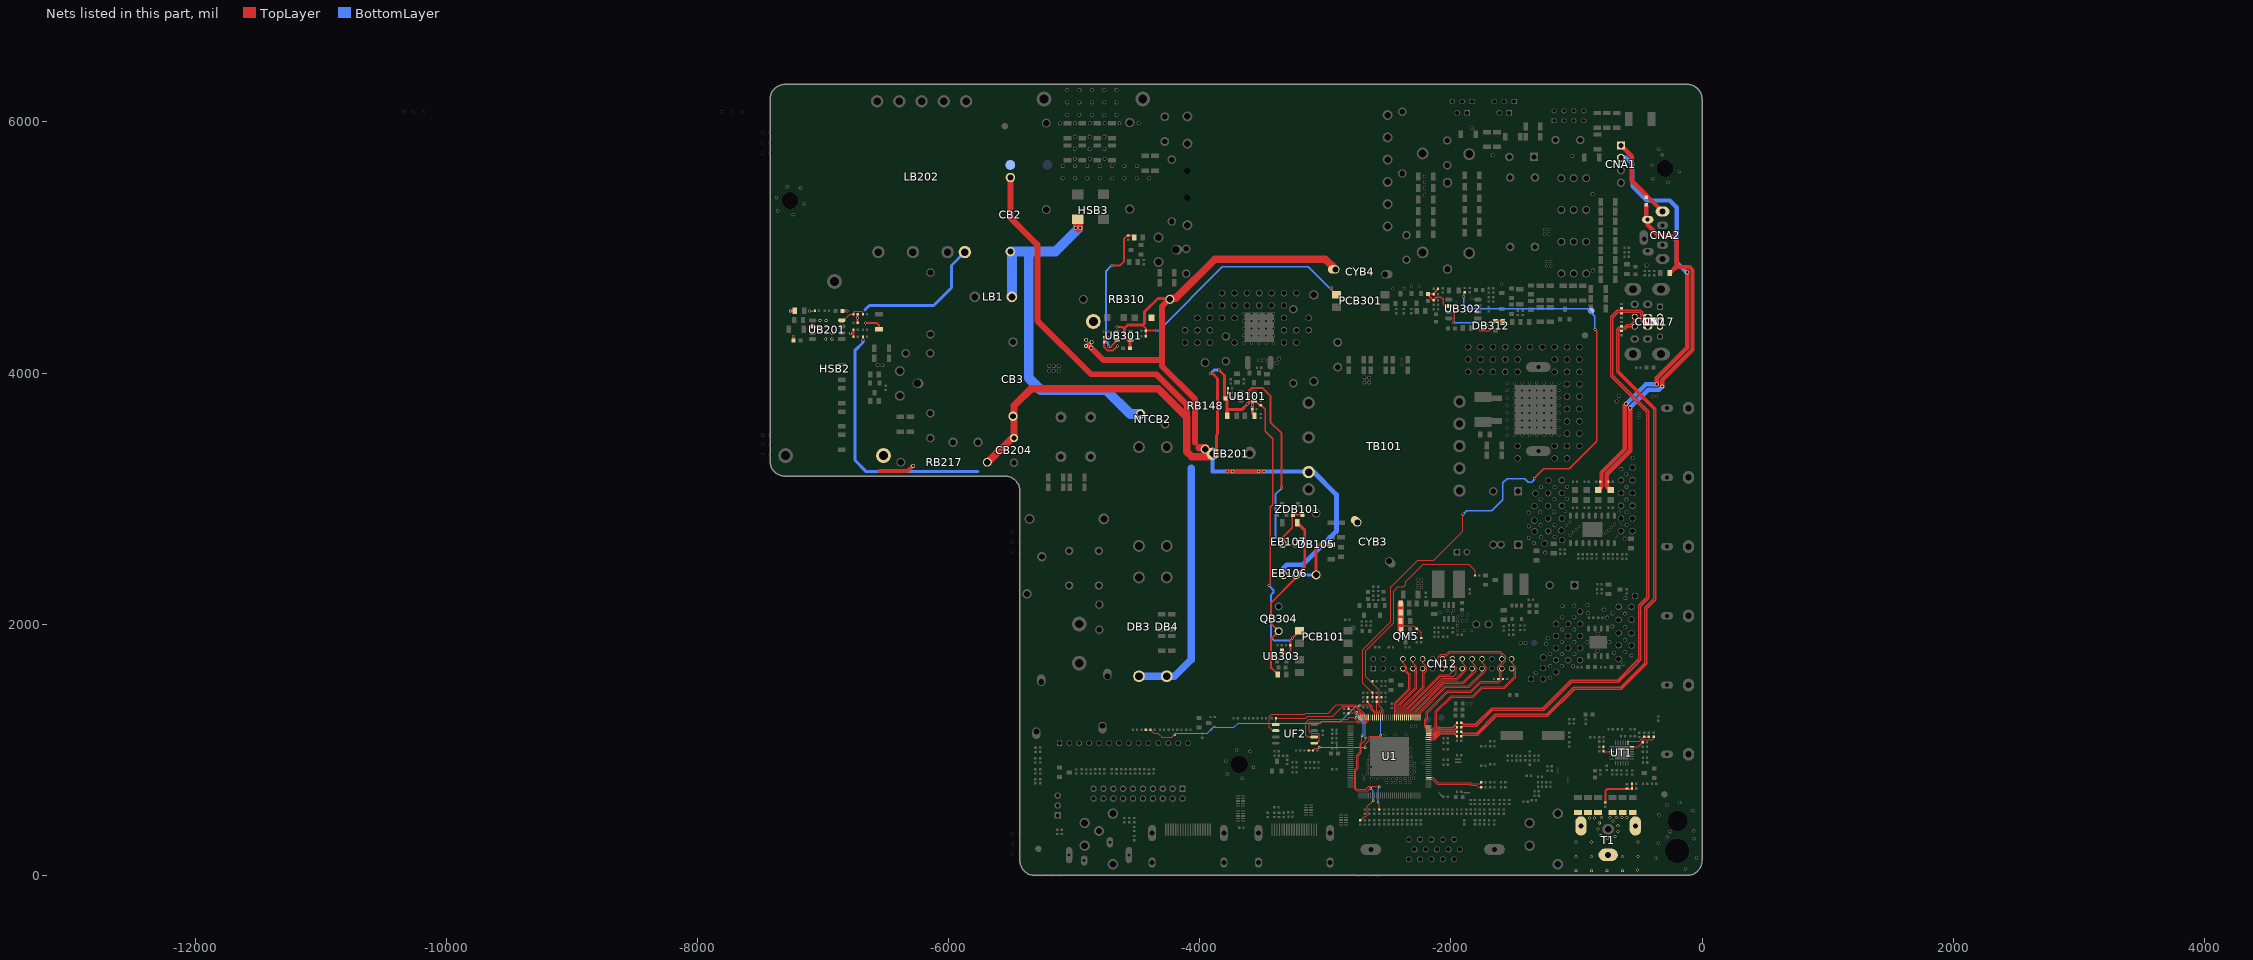
[diagram p0: the nets of this part, all layers, seen from the top]
# Altium PCB MISC84277.PcbDoc (part 13 of 15)
Units mil, origin at the board's own origin, x right, y up, seen from the top; angles counter-clockwise.
Board outline 7422.08 x 6299.21 mil, 2 copper layers (TopLayer, BottomLayer), stack 61.855 mil thick; 709 components, 395 nets, 2812 pads, 811 vias.

## Via types
v1: diameter 23.62, hole 15.75, TopLayer to BottomLayer, tented both sides, 437 vias
v2: diameter 19.68, hole 11.81, TopLayer to BottomLayer, tented both sides, 353 vias
v3: diameter 31.5, hole 23.62, TopLayer to BottomLayer, tented both sides, 16 vias
v4: diameter 31.5, hole 19.68, TopLayer to BottomLayer, tented both sides, 4 vias
v5: diameter 17.72, hole 9.84, TopLayer to BottomLayer, tented both sides, 1 vias

## Nets (pads, with @x,y where several pads share a name; then routed paths per layer and width w, separated by ;. In a path a pad name is that pad's centre, name@x,y a point inside that pad or via, vN(x,y) a via of type N, cw(c..) or ccw(c..) an arc to the next point about the centre after c; other vN are vias at no path point) (continued)
OUT: RB306.1 RB307.1 UB301.6 | length 1145.5
  TopLayer w15.75: v1(-4726.37,4210.62) -4724.41,4208.66 -4709.38,4208.66 UB301.6@-4658.19,4259.84 ; v1(-4700.79,4858.27) -4633.86,4858.27 -4602.36,4889.76 -4602.36,5071.02 RB307.1@-4577.15,5096.23 ; RB307.1@-4569.47,5096.23 -4540.8,5096.23 RB306.1@-4524.06,5079.5
  BottomLayer w15.75: v1(-4726.37,4210.62) -4726.37,4224.4 -4746.06,4244.09 -4746.06,4812.99 v1(-4700.79,4858.27)
OVP: CB322.2 CB323.2 CB324.2 CB328.1 DB312.2 RB351.2 UB302.6 | length 999.2
  TopLayer w11.81: CB322.2@-2177.81,4630.31 CB322.2@-2184,4630.31 ; CB323.2@-2137.23,4629.5 CB323.2@-2137.23,4632.9 ; CB323.2@-2136.73,4632.9 CB323.2@-2137.23,4632.9 ; RB351.2@-2103.84,4668.53 -2137.23,4635.13 CB323.2@-2137.23,4632.9 ; UB302.6@-2046.5,4536 -2062.84,4552.34 -2062.84,4587.34 -2080.25,4604.75 -2117.39,4604.75 -2136.23,4585.9 CB324.2@-2136.23,4581 -2139.15,4581 -2184,4625.85 CB322.2@-2184,4630.31 ; UB302.6@-2017.56,4536 -1991.5,4536 -1974.13,4518.63 -1974.13,4407.87 v1(-1980,4402) ; v1(-1780,4401.5) -1780,4350.5 -1768,4338.5 -1695.5,4338.5 -1680,4354 -1680,4380 DB312.2@-1645.5,4414.5 -1643,4417 -1596.03,4417 CB328.1@-1586.53,4407.5 ; CB322.2@-2184,4630.31 -2181.41,4632.9 CB323.2@-2137.23,4632.9
  BottomLayer w11.81: v1@-1979.66,4402.34 v1@-1780.84,4402.34
PC_LIN: CV6.2 U1.38 | length 444.7
  TopLayer w7: U1.38@-2178.42,781.32 -2145.35,781.32 -2100.56,736.53 -1839.56,736.53 -1833.53,730.5 -1768.23,730.5 CV6.2@-1758.73,739.99
PC_RIN: CV5.2 U1.37 | length 451.4
  TopLayer w7: U1.37@-2178.42,765.57 -2148.57,765.57 -2107.53,724.53 -1844.53,724.53 -1838.5,718.5 -1797.28,718.5 -1779.78,701 CV5.2@-1758.73,701 ; CV5.2@-1761,701 CV5.2@-1758.73,701 ; CV5.2@-1758.73,703.73 CV5.2@-1758.73,701
PFC_CS: CB205.2 RB215.1 UB201.4 | length 225.8
  TopLayer w7.87: UB201.4@-6851.71,4420.37 -6834.63,4420.37 -6786.21,4468.79 CB205.2@-6757.93,4468.79 -6757.93,4482.57 -6747.5,4493 -6692,4493 -6683.12,4484.12 RB215.1@-6683.12,4468.8
PVCC: CM3.2 CM5.2 QM5.S R5V.2 R12V.2 RM5.2 | length 440
  TopLayer w6: -2397.94,1988.24 -2297.24,1988.24 -2272.73,1963.73 -2267.73,1963.73 -2235,1931 RM5.2@-2235,1890.73
  TopLayer w50: R12V.2@-2399.61,2165.35 QM5.S@-2399.4,1952.24
PWM0: RF13.1 RG2.1 U1.86 | length 165.6
  TopLayer w6: RG2.1@-2591.27,1417 -2591.27,1307.54 -2576.05,1292.32 U1.86@-2576.05,1257.7
PWM1: RF18.1 RG1.2 U1.87 | length 191
  TopLayer w6: RG1.2@-2665.27,1417 -2665.27,1384.27 -2627,1346 -2627,1325.56 -2591.8,1290.36 U1.87@-2591.8,1257.7 U1.87@-2590.89,1258.61
PWM_REF: CG2.1 PWM_REF.1 RB366.2 RG2.2 | length 5499.1
  TopLayer w6: RG2.2@-2624.73,1417 CG2.1@-2624.73,1454 -2627,1454 -2701.27,1528.27 -2701.27,1798.4 -2479,2020.67 -2479,2295.92 -2264.92,2510 -2137.83,2510 -1905.51,2742.32 v1(-1905.51,2875.98)
  TopLayer w11.81: v1(-1898.5,4610) -1898.5,4634.27 RB366.2@-1889,4643.77 ; v1(-1336.61,3161.41) -1259.83,3238.19 -1058.78,3238.19 -838.59,3458.39 -838.59,4332.68 v1(-854.33,4348.43)
  BottomLayer w11.81: v1(-1905.51,2875.98) -1875.9,2905.6 -1674.2,2905.6 -1588.1,2991.7 -1588.1,3125.8 -1553.6,3160.3 -1412.8,3160.3 -1382.8,3130.3 -1356.3,3130.3 -1336.61,3149.99 v1(-1336.61,3161.41) ; v1(-1898.5,4610) -1898.5,4547.11 -1864.21,4512.82 -914.39,4512.82 -854.33,4452.76 v1(-854.33,4348.43)
PWR_ON/OFF: RM3.2 RM4.2 RM8.1 U1.84 | length 1985.9
  TopLayer w6: -2572,1417 RM3.2@-2553.73,1417 ; U1.84@-2544.56,1257.7 -2544.56,1287.26 -2540.27,1291.54 -2540.27,1316.27 -2573,1349 -2573,1476 -2679.27,1582.27 -2679.27,1789.29 -2457,2011.56 -2457,2263.47 -2423.32,2297.15 -2376.08,2297.15 -2360.24,2312.99 -2360.24,2336.42 -2219.66,2477 -1859,2477 -1807.73,2425.73 RM4.2@-1807.73,2388
REMOTE: CK6.2 RK16.1 U1.88 | length 2045.2
  TopLayer w6: RK16.1@-4431.56,1160.01 CK6.2@-4393.63,1160.01 -4366.72,1133.1 -4336.05,1133.1 -4301.05,1098.1 -4222.7,1098.1 v2(-4201.3,1119.5) ; v2(-2729,1351) -2721,1359 -2655.56,1359 -2638,1341.44 -2638,1321 -2607.55,1290.55 U1.88@-2607.55,1257.7 U1.88@-2608.3,1258.45
  BottomLayer w6: v2(-4201.3,1119.5) -4189.13,1131.67 -4034.1,1131.67 ; -4047.3,1131.67 -4034.1,1131.67 ; v2(-2729,1351) -2756,1351 -2879,1228 -3027.36,1228 -3042.36,1213 -3695.6,1213 -3730.24,1178.36 -3893.19,1178.36 -3939.87,1131.67 -4034.1,1131.67
RESET-H: U1.89 | length 0.9
  TopLayer w6: U1.89@-2623.3,1257.7 U1.89@-2622.66,1258.34
RF_INPUT: CT13.1 CT40.2 LT3.1 LT11.1 | length 350.1
  TopLayer w15.8: CT40.2@-770.21,579.99 -770.21,662.29 cw(c-741.83,662.29) -761.9,682.36 cw(c-744.86,665.32) -744.86,689.41 -560.31,689.41 LT3.1@-557.46,692.26 CT13.1@-557.46,730.28
RFGND: CT41.2 CT42.2 CT43.2 CT44.2 CT45.2 CT46.2 T1.2 T1.3 T1.4
  other v1: -1006,36.65 -881.75,36.65 -757.5,36.65 -633.25,36.65 -515,41 -1006,152 -881.75,152 -633.25,152 -509,152 -1006,267.35 -881.75,267.35 -509,267.35 -753,295 -695,310 -807,316 -669,348 -830,369 -670,395 -815,418 -708,434 -898,457 -857,458 -801,459 -682,460 -639,460 -598,460 -734,461
ROUT+: CA10.1 CA40.2 CNA2.4 LBA4.2 pad.VIA5@-317.13,3893.19 pad.VIA5@-572.38,3725.25 RA17.1 | length 2944.6
  TopLayer w35: -759,3134.02 -759,3099 LBA4.2@-728,3068 ; -759,3137 -759,3194 -571.5,3381.5 pad.VIA5@-571.5,3723.5 ; CNA2.4@-444.88,5226.4 RA17.1@-444.88,5333.9 ; CNA2.4@-433.07,5222.44 -433.07,5180.2 -348.87,5096 -244.09,5096 -200.89,5052.79 -200.89,4851.88 CA40.2@-256.26,4796.5 ; pad.VIA5@-317.13,3893.19 -317.13,3944.09 -76,4185.22 -76,4821.5 -99.5,4845 -200.89,4845
  BottomLayer w35: pad.VIA5@-572.38,3725.25 -429.63,3868 -342.31,3868 pad.VIA5@-317.13,3893.19
ROUT+': CNA1.1 CNA2.6 RA17.2 | length 678.2
  TopLayer w35: CNA1.1@-646.5,5799.2 CNA1.1@-646.5,5813.67 -560,5727.17 -560,5652.29 -559.5,5651.79 -559.5,5531.5 CNA2.6@-319.34,5291.34
  TopLayer w40: CNA2.6@-319.34,5291.34 CNA2.6@-314.96,5291.34
  BottomLayer w40: CNA2.6@-314.96,5291.49 CNA2.6@-314.96,5293
ROUT-: CA17.1 CNA1.2 LBA3.2 pad.VIA5@-119,4802 pad.VIA5@-360.13,3911 pad.VIA5@-602.2,3756.25 | length 3413.4
  TopLayer w35: LBA3.2@-827,3068 -801,3094 -801,3208.57 -614.5,3395.07 -614.5,3743.94 pad.VIA5@-602.26,3756.19 ; pad.VIA5@-360.13,3911 -360.13,3961.9 -157.76,4164.26 ; -144.26,4177.76 -157.76,4164.26 ; -119,4774.19 -119,4722 ; pad.VIA5@-119,4802 -119,4722 ; -157.76,4164.26 -119,4203.03 -119,4722
  BottomLayer w35: CNA1.2@-646.5,5714.46 -605.66,5714.46 -554,5662.8 -554,5487 -441.27,5374.27 -256.99,5374.27 -202,5319.28 -202,4879.28 -124.72,4802 pad.VIA5@-119,4802 ; pad.VIA5@-600.47,3757.97 -447.44,3911 pad.VIA5@-360.13,3911
RXE0+: CN12.20 U1.69 | length 723.9
  TopLayer w7: U1.69@-2308.34,1257.7 -2308.34,1313.66 -2063,1559 -1951.72,1559 -1877.96,1632.75 -1877.96,1659.37 -1910.08,1691.49 CN12.20@-1910.08,1724.8
RXE0-: CN12.19 U1.70 | length 634.3
  TopLayer w7: U1.70@-2324.08,1257.7 -2324.08,1314.89 -2067.97,1571 -1956.69,1571 -1910.08,1617.6 CN12.19@-1910.08,1646.06 CN12.19@-1903.54,1639.52
RXE1+: CN12.22 U1.67 | length 767.9
  TopLayer w7: U1.67@-2276.84,1257.7 -2276.84,1303.16 -2052,1528 -1899,1528 -1799.22,1627.78 -1799.22,1659.37 -1831.34,1691.49 CN12.22@-1831.34,1724.8
RXE1-: CN12.21 U1.68 | length 680.6
  TopLayer w7: U1.68@-2292.59,1257.7 -2292.59,1304.38 -2056.97,1540 -1903.97,1540 -1831.34,1612.63 CN12.21@-1831.34,1646.06 CN12.21@-1842.91,1646.06
RXE2+: CN12.24 U1.65 | length 828.1
  TopLayer w7: U1.65@-2245.34,1257.7 -2245.34,1292.75 -2040.59,1497.5 -1954,1497.5 ; -1976,1497.5 -1954,1497.5 ; CN12.24@-1752.6,1724.8 -1752.6,1691.49 -1720.48,1659.37 -1720.48,1632.76 -1855.74,1497.5 -1954,1497.5
RXE2-: CN12.23 U1.66 | length 731.3
  TopLayer w7: U1.66@-2261.09,1280.91 U1.66@-2261.09,1257.7 ; U1.66@-2260.5,1258.29 U1.66@-2261.09,1257.7 ; CN12.23@-1752.6,1646.06 -1752.6,1617.6 -1860.71,1509.5 -2045.56,1509.5 -2261.09,1293.97 U1.66@-2261.09,1257.7
RXE3+: CN12.30 U1.61 | length 1193.6
  TopLayer w7: -2151.77,1143.53 U1.61@-2178.42,1143.53 -2151.47,1143.53 -2112,1183 -2112,1302 -1994.5,1419.5 -1821.44,1419.5 -1750.18,1490.76 -1569.9,1490.76 -1484.26,1576.4 -1484.26,1643 ; CN12.30@-1516.38,1724.8 -1516.38,1691.49 -1484.26,1659.37 -1484.26,1643 ; -1484.26,1580.9 -1484.26,1643
RXE3-: CN12.29 U1.62 | length 1046.8
  TopLayer w7: U1.62@-2174.48,1159.27 -2152.7,1159.27 -2124,1187.97 -2124,1306.97 -1999.47,1431.5 -1826.41,1431.5 -1755.15,1502.76 -1574.87,1502.76 -1496.52,1581.11 -1496.52,1626.2 ; CN12.29@-1516.38,1641.19 CN12.29@-1516.38,1646.06 -1496.52,1626.2 ; -1496.52,1585.61 -1496.52,1626.2 ; -1496.52,1620.4 -1496.52,1626.2
RXEC+: CF36.1 CN12.16 CN12.28 U1.63 | length 1570.5
  TopLayer w7: U1.63@-2178.42,1175.02 -2200.61,1175.02 -2210.54,1184.95 -2210.54,1245.41 -2198.2,1257.75 -2198.2,1301.71 -2029.41,1470.5 -1842.56,1470.5 -1768.66,1544.4 -1625.7,1544.4 -1611.5,1558.6 -1611.5,1616.2 -1627.2,1631.9 -1627.2,1660.6 -1595.12,1692.68 CN12.28@-1595.12,1724.8 -1595.12,1755.75 -1612.67,1773.3 -2009.53,1773.3 -2035.24,1747.6 -2049.1,1747.6 -2067.56,1729.14 CN12.16@-2067.56,1724.8
RXEC-: CF35.2 CN12.15 CN12.27 U1.64 | length 1719.5
  TopLayer w7: U1.64@-2192.74,1190.77 U1.64@-2178.42,1190.77 -2196.68,1190.77 -2198.54,1192.63 -2198.54,1240.44 -2186.2,1252.78 -2186.2,1296.74 -2024.44,1458.5 -1837.59,1458.5 -1763.69,1532.4 -1620.73,1532.4 -1599.5,1553.63 -1599.5,1671.33 -1562.5,1708.33 -1562.5,1740.1 -1607.7,1785.3 -2014.51,1785.3 -2040.21,1759.6 -2077.5,1759.6 -2099.4,1737.7 -2099.4,1710.9 -2067.56,1679.06 CN12.15@-2067.56,1646.06
RXO0+: CN12.8 U1.77 | length 537
  TopLayer w7: U1.77@-2434.32,1257.7 -2434.32,1370.68 -2324,1481 -2324,1601 -2350.4,1627.4 -2350.4,1659.37 -2382.52,1691.49 CN12.8@-2382.52,1724.8
RXO0-: CN12.7 U1.78 | length 454.9
  TopLayer w7: U1.78@-2450.07,1257.7 -2450.07,1284.4 -2446.32,1288.15 -2446.32,1375.65 -2336,1485.97 -2336,1596.03 -2382.52,1642.55 CN12.7@-2382.52,1646.06
RXO1+: CN12.10 U1.75 | length 534.7
  TopLayer w7: U1.75@-2402.83,1257.7 -2402.83,1357.17 -2271.66,1488.34 -2271.66,1659.37 -2303.78,1691.49 CN12.10@-2303.78,1724.8
RXO1-: CN12.9 U1.76 | length 464.5
  TopLayer w7: U1.76@-2418.57,1257.7 -2418.57,1358.4 -2283.66,1493.31 -2283.66,1625.94 CN12.9@-2303.78,1646.06 CN12.9@-2291.86,1646.06
RXO2+: CN12.12 U1.73 | length 554.3
  TopLayer w7: U1.73@-2371.33,1257.7 -2371.33,1340.67 -2213.04,1498.96 -2213.04,1607.96 -2192.92,1628.08 -2192.92,1659.37 -2225.04,1691.49 CN12.12@-2225.04,1724.8
RXO2-: CN12.11 U1.74 | length 455.5
  TopLayer w7: U1.74@-2387.08,1257.7 -2387.08,1341.89 -2225.04,1503.93 CN12.11@-2225.04,1646.06
RXO3+: CN12.18 U1.71 | length 698.9
  TopLayer w7: U1.71@-2339.83,1257.7 -2339.83,1326.17 -2080,1586 -1978,1586 -1956.7,1607.3 -1956.7,1659.36 -1988.82,1691.49 CN12.18@-1988.82,1724.8
RXO3-: CN12.17 U1.72 | length 581.9
  TopLayer w7: U1.72@-2355.51,1257.77 U1.72@-2355.58,1257.7 -2355.58,1327.39 -2084.97,1598 -2014,1598 -1988.82,1623.18 CN12.17@-1988.82,1646.06
SGND: CB2.2 CB3.2 CB101.2 CB102.2 CB103.2 CB111.1 CB112.1 CB201.1 CB204.1 CB205.1 CB206.1 CB212.2 CB221.1 CB301.1 CB303.2 CB304.2 CYB3.1 CYB4.1 DB3.A DB4.A DB371.K EB106.2 EB107.2 EB201.2 HSB2.3@-6519.24,3343.09 HSB3.1 LB202.6@-5871.51,4963.91 pad.VIA5@-3488.19,3216.54 pad.VIA5@-3533.46,3216.09 pad.VIA5@-3740.16,3216.09 pad.VIA5@-4862.5,4245.5 pad.VIA5@-4866.6,4203.6 pad.VIA5@-4905.8,4265.5 pad.VIA5@-4906.5,4215.9 pad.VIA5@-6283.46,3261.81 pad.VIA5@-6929.56,4319.62 pad.VIA5@-6930.47,4270.7 pad.VIA5@-6976.67,4418.38 pad.VIA5@-6977.58,4369.46 pad.VIA5@-6978.49,4320.53 pad.VIA5@-6979.39,4271.61 pad.VIA5@-7025.59,4419.29 pad.VIA5@-7026.5,4370.37 PCB101.3 PCB301.3 RB103.1 RB104.1 RB148.1 RB205.1 RB206.2 RB217.1 RB218.1 RB226.1 RB227.1 RB302.2 RB303.2 RB304.2 RB310.1 TB101.5 TP-TDT.2 UB101.1 UB201.6 UB301.1 UB303.A ZDB101.1 ZDB101.3 | length 26092.7
  TopLayer w7.87: CB205.1@-6724.6,4468.65 CB205.1@-6724.46,4468.79
  TopLayer w11.81: v1(-7108.13,4494.01) -7068.03,4494.01 RB227.1@-7065.69,4496.35 RB227.1@-7067.3,4497.97 ; CB201.1@-6843.74,4496.35 -6812.87,4496.35 v1(-6811.03,4494.51) ; CB102.2@-3796.31,3798 -3776.23,3818.08 CB101.2@-3776.23,3879.5 ; UB101.1@-3582.22,3777.1 UB101.1@-3565.35,3777.1 -3558.59,3777.1 -3524.76,3743.27 -3509.8,3743.27 -3480.32,3713.79 -3480.32,3537.39 -3419.31,3476.38 -3419.31,2950.77 -3439.1,2930.98 -3439.1,2322.71 -3452.76,2309.06 v1(-3450.78,2309.05) ; v1(-2953.5,4677) -2953.5,4662 -2916,4624.5 PCB301.3@-2910.13,4624.5
  TopLayer w15.75: CB206.1@-7237.65,4257.84 v1(-7237.65,4292.85) ; v1(-6782,4317.5) -6757.93,4317.5 ; RB205.1@-6757.93,4290 -6757.93,4317.5 ; RB206.2@-6757.93,4345.31 -6757.93,4317.5 ; CB205.1@-6724.6,4468.65 -6724.46,4468.51 RB226.1@-6724.46,4400.61 ; CB221.1@-6683.12,4290.01 -6683.12,4262.12 v1(-6683,4262) ; v1(-6661,4399) -6572,4399 -6555,4382 RB218.1@-6555,4350.89 ; CB303.2@-4762.14,4287.55 RB303.2@-4762.14,4244.24 -4762.14,4206.04 -4736.45,4180.35 -4691.02,4180.35 v1(-4654.83,4216.54) ; v1(-4661.42,4366.14) -4616.14,4366.14 -4608.27,4358.27 ; -4456.69,4381.89 -4430.35,4355.54 RB304.2@-4430.35,4338.63 ; CB301.1@-4430.35,4295.33 RB304.2@-4430.35,4338.63 ; v1(-4346.51,4338.63) RB304.2@-4430.35,4338.63 ; -3608.27,3765.75 -3608.27,3860.24 -3588.58,3879.92 -3500,3879.92 -3438.73,3818.65 -3438.73,3609.99 -3348.43,3519.68 v1(-3348.43,3084.65) ; UB303.A@-3346,1783.5 -3337,1774.5 -3289,1774.5 -3279.77,1783.73 RB302.2@-3279.77,1832.5 -3279.77,1872.23 v1(-3261,1891) -3261,1893.63 PCB101.3@-3205.13,1949.5 ; EB107.2@-3332.21,2640.07 -3332.21,2699.29 -3264,2767.5 -3264,2868 ZDB101.1@-3256.5,2875.5 ZDB101.3@-3181.5,2875.5
  TopLayer w23.62: v1(-7261.85,4496.35) CB212.2@-7224.78,4496.35 ; CB304.2@-4556.33,4197.94 -4556.33,4246.2 -4600.39,4290.27 -4600.39,4358.27 -4576.77,4381.89 -4456.69,4381.89 -4438.98,4399.61 -4438.98,4490.16 -4334.13,4595 RB310.1@-4238.12,4595 ; v1(-3915.35,3996.06) -3897.64,3996.06 -3858.39,3956.82 -3858.39,3513.65 -3868.11,3503.94 -3868.11,3386.72 EB201.2@-3897.83,3357 ; v1(-3848.73,4025.46) -3848.3,4025.46 -3803.02,3980.19 -3803.02,3816.93 -3803.02,3797.12 -3782.03,3776.13 -3782.03,3708.66 ; CB112.1@-3782.03,3660.5 -3782.03,3708.66 ; UB101.1@-3582.22,3777.1 -3596.92,3777.1 -3608.27,3765.75 v1(-3621.06,3752.95) -3665.35,3708.66 -3782.03,3708.66 ; UB101.1@-3581.73,3776.61 v1(-3581.73,3746.06) RB104.1@-3581.73,3713.5 -3581.73,3682.13 -3564.47,3664.86 CB111.1@-3564.47,3660
  TopLayer w27.56: UB201.6@-7084,4370.37 pad.VIA5@-7026.5,4370.37
  TopLayer w31.5: -6551.34,3218.66 -6326.61,3218.66 pad.VIA5@-6283.46,3261.81 ; v1(-3779.52,3216.09) -3488.64,3216.09 pad.VIA5@-3488.19,3216.54
  TopLayer w47.24: CB2.2@-5509,5557.78 -5509,5237.35 -5294.5,5022.85 -5294.5,4418.1 ; -5263.01,4386.61 -5294.5,4418.1 ; -4887.9,4223.8 -4767.2,4103.1 -4301.18,4103.1 ; -4297.24,3940.94 -4270.65,3914.35 ; RB310.1@-4238.12,4595 -4301.18,4531.94 -4301.18,4103.1 ; -4103.82,3647.13 -4103.82,3747.52 -4270.65,3914.35 ; -4037.13,3448.82 -4037.13,3791.06 -4301.18,4055.12 -4301.18,4103.1 ; -5294.5,4418.1 -4867.2,3990.8 -4347.1,3990.8 -4270.65,3914.35
  TopLayer w59.06: RB217.1@-5692.01,3290.5 -5687.85,3290.5 -5494.98,3483.37 CB204.1@-5480.13,3483.37 -5480.13,3738.97 -5343.7,3875.4 -4332.09,3875.4 -4103.82,3647.13 -4103.82,3374.5 -4062.82,3333.5 -3921.33,3333.5 EB201.2@-3897.83,3357 ; RB310.1@-4238.12,4595 -4192.4,4595 -3879.62,4907.78 -3000.94,4907.78 CYB4.1@-2918.85,4825.69 ; -4003.14,3404.51 RB148.1@-3952.48,3404.51
  BottomLayer w11.81: v1(-4346.51,4338.63) -4328.69,4338.63 -3820.87,4846.46 -3135.83,4846.46 -2966.37,4677 v1(-2953.5,4677)
  BottomLayer w15.75: v1@-6683.5,4262 v1(-6683,4262) ; v1(-3450.78,2309.05) -3413.39,2271.66 -3413.39,2252.71 -3432.32,2233.78 -3432.32,1892.34 -3411.23,1871.25 -3280.75,1871.25 v1(-3261,1891) ; v1(-3348.43,3084.65) -3397.64,3035.43 -3397.64,2705.5 EB107.2@-3332.21,2640.07
  BottomLayer w23.62: v1(-6683,4262) -6683,4244.5 -6745,4182.5 -6745,3303 -6657,3215 -5767.51,3215 ; -6666.5,4504 -6632.62,4537.88 -6119.9,4537.88 -5977.69,4680.09 -5977.69,4857.73 LB202.6@-5871.51,4963.91 ; LB202.6@-5890.51,4968.41 LB202.6@-5890.51,4987.12 ; v1(-3915.35,3996.06) -3885.95,4025.46 v1(-3848.73,4025.46)
  BottomLayer w31.5: EB201.2@-3897.83,3357 -3897.83,3216.72 -3897.19,3216.09 v1(-3779.52,3216.09) -3137.37,3216.09 TB101.5@-3133.09,3211.81
  BottomLayer w39.37: EB106.2@-3332.46,2390.43 -3332.7,2390.67 -3332.7,2447.3 -3306.5,2473.5 -3179,2473.5 -2912.5,2740 -2912.5,3031.5 -3092.81,3211.81 TB101.5@-3133.09,3211.81
  BottomLayer w47.24: CB2.2@-5509,5557.78 CB2.2@-5501.14,5565.64
  BottomLayer w59.06: DB3.A@-4484.49,1585.72 -4201.61,1585.72 -4068.61,1718.72 -4068.61,3242.41
  other v1: -6724.6,4437.1
SPDIF_OUT: CO8.1 RO9.1 U1.85 | length 885.5
  TopLayer w6: v2(-2684.2,1015.1) -2684.2,1043.42 -2650.98,1076.64 -2650.98,1103.53 -2646.02,1108.5 v2@-2564.5,1108.5 ; U1.85@-2560.31,1257.7 v1@-2560.31,1304.14
  TopLayer w8: RO9.1@-3133.27,994.42 CO8.1@-3097.73,994.42 -3078.89,1013.26 -3056.54,1013.26 v2(-3048.8,1021) v2@-3048.8,1015.11
  BottomLayer w6: v2@-2560.08,1116.08 v1(-2560.08,1304.37)
  BottomLayer w8: v2(-3048.8,1021) v2@-2690.1,1021
  other v2: -2560,1116
SPI_CLK: U1.92 UF2.6 | length 717.5
  TopLayer w6: -3126.06,1103 -3142.23,1103 -3157,1117.77 -3157,1216.11 -3129.11,1244 -2823,1244 -2818.84,1248.16 -2818.84,1248.39 -2808.39,1258.84 -2776.48,1258.84 -2743.64,1226 -2679.56,1226 -2670.54,1235.01 U1.92@-2670.54,1257.7
  TopLayer w15: -3126.06,1102.34 -3088.8,1102.34 UF2.6@-3088.46,1102
SPI_CSN: RF3.1 U1.94 UF2.1 | length 831.4
  TopLayer w6: UF2.1@-3395.54,1202 -3394.27,1203.28 RF3.1@-3394.27,1251 -3157,1251 -3142,1266 -2941.44,1266 -2861.44,1346 -2767,1346 -2702.04,1281.04 U1.94@-2702.04,1257.7
SPI_DI: U1.91 UF2.5 | length 764.4
  TopLayer w6: -3053.68,1069.32 -3048,1075 -3048,1119 -3059,1130 -3112.19,1130 -3129,1146.81 -3129,1213 -3120,1222 -2755.19,1222 -2748.19,1215 -2675,1215 -2654.79,1235.21 U1.91@-2654.79,1257.7
  TopLayer w15: UF2.5@-3088.46,1052 -3071,1052 -3053.68,1069.32
SPI_DO: U1.93 UF2.2 | length 999.3
  TopLayer w6: UF2.2@-3395.54,1152 -3417.57,1152 -3446.6,1181.03 -3446.6,1262.15 -3426.9,1281.84 -3165.01,1281.84 -3155.51,1291.34 -2978.35,1291.34 -2912.69,1357 -2761,1357 -2686.29,1282.29 U1.93@-2686.29,1257.7
T-IF-AGC: CT1.2 RT2.2 UT1.15 | length 118.5
  TopLayer w6: UT1.15@-720.73,985.26 UT1.15@-720.63,985.15
  TopLayer w8: CT1.2@-785.62,989.64 RT2.2@-785.62,1025.41 RT2.2@-785.39,1025.18 ; CT1.2@-785.39,989.41 -781.13,985.15 UT1.15@-720.63,985.15 UT1.15@-736.36,985.15
TUNER_SCL: CT8.2 RT6.2 UT1.6 | length 224.6
  TopLayer w6: UT1.6@-559.21,1024.52 -507.31,1024.52 -473.42,1058.41 -473.42,1071.61 -464.62,1080.41 -395.62,1080.41 -385.62,1090.41 RT6.2@-385.62,1101.2 ; RT6.2@-385.62,1103.68 RT6.2@-385.62,1101.2 ; RT6.2@-383.7,1103.13 RT6.2@-385.62,1101.2
TUNER_SDA: CT7.2 RT5.2 UT1.7 | length 193.1
  TopLayer w6: UT1.7@-590.71,1056.02 -590.71,1066.09 -587.31,1069.49 -499.55,1069.49 -465.91,1103.13 RT5.2@-422.97,1103.13
UART_RX: RF8.1 RF11.1 U1.96 | length 1180.1
  TopLayer w6: RF8.1@-2816.27,1291 -2812.43,1294.84 -2773.84,1294.84 -2753.38,1274.38 v2(-2753.38,1260.97) ; v2@-2750.1,1257.7 U1.96@-2733.53,1257.7 U1.96@-2734.63,1258.8 ; RF11.1@-2722,438.73 -2694.73,466 -2679,466 -2667,478 -2667,549.56 v2@-2620.56,596 ; v2@-2710,1112.1 -2710,1066.11 -2724.06,1052.06 -2724.06,982.61 -2748.84,957.83 -2748.84,857.86 -2767.5,839.2 -2767.5,689.24 -2753.26,675 -2657.65,675 v2(-2639.65,693)
  BottomLayer w6: v2@-2743.7,1260.97 -2697.19,1214.46 -2697.19,1124.41 v2@-2709.5,1112.1 ; v2(-2639.65,693) -2618,671.35 v2(-2618,596)
  other v2: -2704.7,1112.2
UART_TX: RF9.1 RF10.1 U1.95 | length 1202.3
  TopLayer w6: RF9.1@-2816.27,1327 -2812.27,1323 -2776.77,1323 v2(-2751.38,1297.62) ; v2@-2750.77,1297 -2733.56,1297 -2717.79,1281.23 U1.95@-2717.79,1257.7 ; v2@-2679.83,1095.1 -2679.83,1078.91 -2713.06,1045.68 -2713.06,978.05 -2737.84,953.27 -2737.84,853.3 -2756.5,834.64 -2756.5,693.8 -2748.7,686 -2679,686 -2654.16,710.84 v2@-2574.74,710.84 ; v2(-2581,581) -2572,572 RF10.1@-2572,524.73 ; v2(-2569.8,705.9) v2@-2574.74,710.84 ; v2@-2568,706 -2572.84,710.84 v2@-2574.74,710.84
  BottomLayer w6: v2(-2751.38,1297.62) -2751.38,1284.21 -2683.16,1215.99 v2@-2683.16,1095.1 ; v2(-2581,581) -2581,690 v2@-2568,703
  other v2: -2680.3,1094
USB0_DM: RU1.1 U1.59 | length 254.3
  TopLayer w7: U1.59@-2178.42,1112.03 -2148.59,1112.03
  TopLayer w10: -2148.59,1111.78 -2142.92,1111.78 -2093.69,1161 -1969.23,1161 RU1.1@-1951.73,1178.5
USB0_DP: RU3.1 U1.60 | length 263.7
  TopLayer w7: U1.60@-2178.42,1127.78 -2146.28,1127.78
  TopLayer w10: -2146.28,1129.63 -2099.91,1176 -1987.08,1176 -1951.73,1211.34 RU3.1@-1951.73,1214.5
USB0_M: CN5.6 CN7.2@-433.46,4370.08 CN17.3 DU3.K RU1.2 | length 5038.5
  TopLayer w11: RU1.2@-1918.27,1178.5 -1908.77,1188 -1798.38,1188 -1669.62,1316.76 -1260.97,1316.76 -1039.39,1538.34 -665.82,1538.34 -533.67,1670.5 ; -528.58,1675.58 -533.67,1670.5 ; CN7.2@-433.46,4370.08 -433.46,4400.04 ; CN17.3@-335.48,4369.63 -366.35,4400.5 -469,4400.5 -489.5,4421 -489.5,4476.37 -499.63,4486.5 -668.37,4486.5 -713,4441.87 -713,3982.9 -424.5,3694.4 -424.5,2207.55 -487.24,2144.81 -487.24,1716.92 -533.67,1670.5
USB0_P: CN5.7 CN7.3 CN17.2 DU4.K RU3.2 | length 5048.8
  TopLayer w11: RU3.2@-1918.27,1214.5 -1914.5,1214.5 -1904,1204 -1805.01,1204 -1676.25,1332.76 -1267.6,1332.76 -1046.02,1554.34 -672.45,1554.34 -503.24,1723.55 -503.24,2151.44 -440.5,2214.18 -440.5,3687.77 -729,3976.27 -729,4448.5 -675,4502.5 -493,4502.5 -473.5,4483 -473.5,4427.63 -462.37,4416.5 -367.35,4416.5 CN17.2@-335.48,4448.37 ; -433.46,4419.96 CN7.3@-433.46,4448.82 CN7.3@-433.46,4431.04
USB1_DM: RU2.1 U1.57 | length 254.5
  TopLayer w7: U1.57@-2178.42,1080.53 -2145,1080.53
  TopLayer w10: -2145,1079.78 -2132.49,1079.78 -2085.27,1127 -1971.73,1127 RU2.1@-1951.73,1107
USB1_DP: RU4.1 U1.58 | length 246.2
  TopLayer w7: U1.58@-2178.42,1096.28 -2147,1096.28
  TopLayer w10: -2147,1095.78 -2137.7,1095.78 -2091.48,1142 -1952.73,1142 RU4.1@-1951.73,1143
USB1_M: CN5.2 DU7.K RU2.2 | length 4667
  TopLayer w11: RU2.2@-1918.27,1107 -1908.27,1117 -1788.77,1117 -1640.01,1265.76 -1231.36,1265.76 -1015.78,1481.34 -642.21,1481.34 -439.24,1684.31 -439.24,2124.93 -367.5,2196.67 -367.5,3718.01 -665,4015.51 -665,4339 -655.5,4348.5 -611.87,4348.5 -590.29,4370.08 CN5.2@-536.61,4370.08
USB1_P: CN5.3 DU8.K RU4.2 | length 4705.5
  TopLayer w11: RU4.2@-1918.27,1143 -1908.27,1133 -1795.4,1133 -1646.64,1281.76 -1237.99,1281.76 -1022.41,1497.34 -648.84,1497.34 -455.24,1690.94 -455.24,2131.56 -387.31,2199.49 ; CN5.3@-536.61,4448.82 -536.61,4418.33 -568.87,4386.08 -596.92,4386.08 -618.5,4364.5 -662.13,4364.5 -681,4345.63 -681,4008.88 -383.5,3711.38 -383.5,2203.3
VBRIDGE: CB2.1 DB202.A LB1.1@-5497.36,4607.5 NTCB2.1 pad.VIA5@-4950.79,5157.48 pad.VIA5@-4988.79,5157.48 | length 3051
  TopLayer w78.74: -4970.47,5159.45 DB202.A@-4970.47,5213.67
  BottomLayer w78.74: LB1.1@-5497.36,4607.5 -5497.36,4955.59 CB2.1@-5509,4967.22 -5385.22,4967.22 ; -5362.5,3961.91 -5267.29,3866.7 -4745.93,3866.7 -4554.57,3675.34 NTCB2.1@-4472.93,3675.34 ; -5362.5,3965.9 -5362.5,4944.5 -5385.22,4967.22 ; -4970.47,5147.64 -5150.89,4967.22 -5385.22,4967.22
VCC1: DB105.K EB106.1 QB304.C RB110.2 RB116.1 RB326.1 | length 1919.2
  TopLayer w15.75: RB326.1@-3379.59,1600 -3432.32,1652.72 -3432.32,1884.76 QB304.C@-3372.5,1944.58 -3432.32,2004.39 -3432.32,2172.01 -3234.04,2370.29 EB106.1@-3234.04,2390.43
  TopLayer w23.62: EB106.1@-3234.04,2390.43 -3164.5,2459.96 -3164.5,2748.05 RB110.2@-3223.95,2807.5 ; DB105.K@-3074,2392.44 -3074,2608.99 -3048.61,2634.38 RB116.1@-2954.39,2634.38
  BottomLayer w23.62: EB106.1@-3232.03,2392.44 DB105.K@-3074,2392.44